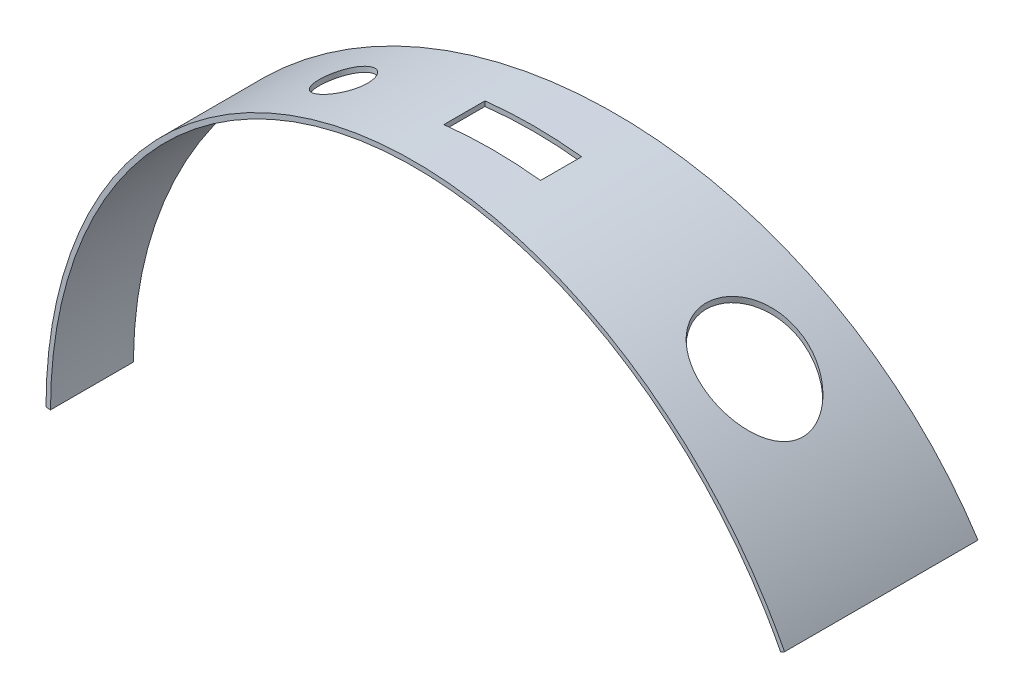
from build123d import *

# Parameters (mm, degrees)
SHEET_EXTRUDE_1_1_BACK   = 40
SHEET_EXTRUDE_1_1_DEPTH  = 80
THICKEN_1_T1             = 1
THICKEN_1_T2             = 1
SKETCH_2_OUTSIDE_W       = 406.64
SKETCH_2_OUTSIDE_H       = 158.22
CUT_EXTRUDE_1_DEPTH      = 253.095220105
CUT_EXTRUDE_2_REACH      = 254.095
CUT_EXTRUDE_2_END_RADIUS = 176
SKETCH_3_W               = 40
SKETCH_3_H               = 17
CUT_EXTRUDE_3_REACH      = 254.095
CUT_EXTRUDE_3_END_RADIUS = 176
SKETCH_4_R               = 20
CUT_EXTRUDE_4_REACH      = 254.095
SKETCH_5_R               = 10


with BuildPart() as body_1:
    # Sheet Extrude 1: a surface, the sketch's curves swept straight by 80 mm
    with BuildLine(Plane.XY.offset(-SHEET_EXTRUDE_1_1_BACK), mode=Mode.PRIVATE) as sheet_extrude_1_1_path:
        ThreePointArc((151.554445662, 87.5), (-45.293332893, 169.037019601), (-175, 0))
    sheet_extrude_1_1 = Shell.extrude(sheet_extrude_1_1_path.wire(), (0 * SHEET_EXTRUDE_1_1_DEPTH, 0 * SHEET_EXTRUDE_1_1_DEPTH, 1 * SHEET_EXTRUDE_1_1_DEPTH))
    add(Solid.thicken(sheet_extrude_1_1, THICKEN_1_T1))
    add(Solid.thicken(sheet_extrude_1_1, -THICKEN_1_T2))

    # 草图2 outside → 切除-拉伸1 (cut, through all)
    with BuildSketch(Plane(origin=(0, 0, 0), x_dir=(1, 0, 0), z_dir=(0, 1, 0))):
        with Locations((-11.79, 0)):
            Rectangle(SKETCH_2_OUTSIDE_W, SKETCH_2_OUTSIDE_H)
        Polygon((152.420471066, 40), (-197.579528934, 15.52561582), (-197.579528934, -15.52561582), (152.420471066, -40), align=None, mode=Mode.SUBTRACT)
    extrude(amount=CUT_EXTRUDE_1_DEPTH, mode=Mode.SUBTRACT)

    # 切除-拉伸2: up to this cylinder (the profile starts inside it)
    cut_extrude_2_end = Plane(origin=(0, 0, 0), z_dir=(0, 0, 1)) * Cylinder(CUT_EXTRUDE_2_END_RADIUS, 861.19, mode=Mode.PRIVATE)
    # 草图3 → 切除-拉伸2 (cut, up to the surface)
    with BuildSketch(Plane(origin=(0, 0, 0), x_dir=(1, 0, 0), z_dir=(0, 1, 0)), mode=Mode.PRIVATE) as cut_extrude_2_sk1:
        Rectangle(SKETCH_3_W, SKETCH_3_H)
    cut_extrude_2_tool1 = extrude(cut_extrude_2_sk1.sketch, amount=CUT_EXTRUDE_2_REACH, mode=Mode.PRIVATE) & cut_extrude_2_end
    add(cut_extrude_2_tool1.solids().sort_by_distance((0, 0, 0))[0], mode=Mode.SUBTRACT)

    # 切除-拉伸3: up to this cylinder (the profile starts inside it)
    cut_extrude_3_end = Plane(origin=(0, 0, 0), z_dir=(0, 0, 1)) * Cylinder(CUT_EXTRUDE_3_END_RADIUS, 861.19, mode=Mode.PRIVATE)
    # 草图4 → 切除-拉伸3 (cut, up to the surface)
    with BuildSketch(Plane(origin=(0, 0, 0), x_dir=(1, 0, 0), z_dir=(0, 1, 0)), mode=Mode.PRIVATE) as cut_extrude_3_sk1:
        with Locations(Location((100, 0, 0), (0, 0, 90))):
            Circle(SKETCH_4_R)
    cut_extrude_3_tool1 = extrude(cut_extrude_3_sk1.sketch, amount=CUT_EXTRUDE_3_REACH, mode=Mode.PRIVATE) & cut_extrude_3_end
    add(cut_extrude_3_tool1.solids().sort_by_distance((100, 0, 0))[0], mode=Mode.SUBTRACT)

    # 草图5 → 切除-拉伸4 (cut, up to next)
    with BuildSketch(Plane(origin=(0, 0, 0), x_dir=(1, 0, 0), z_dir=(0, 1, 0)), mode=Mode.PRIVATE) as cut_extrude_4_sk1:
        with Locations(Location((-70, 0, 0), (0, 0, 90))):
            Circle(SKETCH_5_R)
    cut_extrude_4_tool1 = extrude(cut_extrude_4_sk1.sketch, amount=CUT_EXTRUDE_4_REACH, mode=Mode.PRIVATE) & body_1.part
    add(cut_extrude_4_tool1.solids().sort_by_distance((-70, 0, 0))[0], mode=Mode.SUBTRACT)


solid = body_1.part
